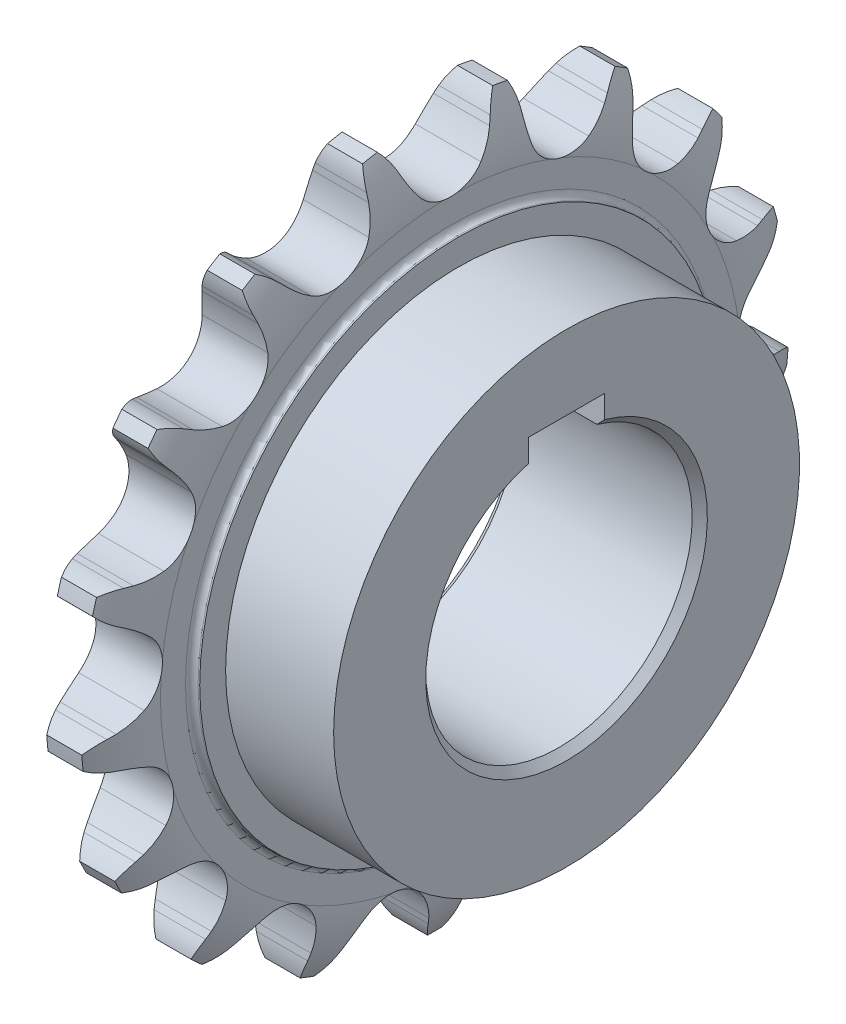
SolidWorks part; units mm, degrees
ref_plane "前视基准面" through (0, 0, 0) normal (0, 0, 1) x (1, 0, 0)
ref_plane "上视基准面" through (0, 0, 0) normal (0, 1, 0) x (1, 0, 0)
ref_plane "右视基准面" through (0, 0, 0) normal (1, 0, 0) x (0, 0, -1)
sketch "草图1" plane through (0, 0, 0) normal (0, 0, 1) x (1, 0, 0)
  line L0 (-7.9375, 0) -> (7.9375, 0) construction
  line L1 (-5.4059, 17.5) -> (-5.4059, 34)
  line L2 (-5.4059, 34) -> (-5.1989, 34)
  line L3 (-4.371, 34.8279) -> (-4.371, 38.1174)
  line L4 (-2.3072, 46.5) -> (2.3072, 46.5)
  line L5 (4.371, 38.1174) -> (4.371, 34.8279)
  line L6 (5.1989, 34) -> (5.4059, 34)
  line L7 (5.4059, 34) -> (5.4059, 17.5)
  line L8 (5.4059, 17.5) -> (-5.4059, 17.5)
  line L9 (0, 0) -> (0, 46.5) construction
  line L10 (-3.7169, 43.1974) -> (3.7169, 43.1974) construction
  line L11 (-3.7169, -43.1974) -> (3.7169, -43.1974) construction
  line L12 (7.9375, 0) -> (24.9375, 0) construction
  line L13 (-4.371, 38.1174) -> (3.7984, 38.1174) construction
  line L14 (-4.371, -38.1174) -> (3.7984, -38.1174) construction
  line L15 (24.9375, 0) -> (35.0975, 0) construction
  line L16 (35.0975, 0) -> (50.1875, 0) construction
  line L17 (50.1875, 0) -> (59.5875, 0) construction
  line L18 (59.5875, 0) -> (77.6975, 0) construction
  arc A0 (-2.3072, 46.5) -> (-4.371, 38.1174) centre (11.4948, 38.6567) ccw
  arc A1 (2.3072, 46.5) -> (4.371, 38.1174) centre (-11.4948, 38.6567) cw
  arc A2 (4.371, 34.8279) -> (5.1989, 34) centre (5.1989, 34.8279) ccw
  arc A3 (-5.1989, 34) -> (-4.371, 34.8279) centre (-5.1989, 34.8279) ccw
  point P30 (4.371, 34)
  point P33 (-4.371, 34)
  dimension "D1" = 4.1174
  dimension "rx" = 15.875
  dimension "D3" = 0.8279
  dimension "d" = 86.3948
  dimension "p" = 15.875
  dimension "z" = 17
  dimension "da" = 93
  dimension "df" = 76.2348
  dimension "dr" = 10.16
  dimension "dk" = 35
  dimension "dg" = 68
  dimension "h" = 15.09
  dimension "bf1" = 8.742
  dimension "b1" = 9.4
  dimension "ba" = 2.0638
  dimension "D2" = 1.0349
  dimension "pt" = 18.11
revolve "旋转1" add sketch "草图1" angle 360 about L0
sketch "草图2" plane through (0, 0, 0) normal (1, 0, 0) x (0, 0, -1)
  line L0 (0, 0) -> (0, 46.5) construction
  line L1 (0, 0) -> (-8.5444, 45.7082) construction
  line L2 (0, 0) -> (-16.7977, 43.36) construction
  line L3 (4.033, 39.986) -> (5.4737, 38.8388) construction
  line L4 (5.7931, 42.895) -> (-6.3584, 48.2605) construction
  line L5 (0, 0) -> (8.5444, 45.7082) construction
  line L6 (5.7931, 42.895) -> (6.1811, 43.7738)
  line L7 (-5.7931, 42.895) -> (-6.1811, 43.7738)
  circle A0 centre (0, 0) radius 46.5 construction
  arc A1 (4.033, 39.986) -> (-4.033, 39.986) centre (0, 43.1974) cw
  arc A2 (4.033, 39.986) -> (5.7931, 42.895) centre (-6.3584, 48.2605) ccw
  arc A3 (7.5795, 45.8781) -> (6.1811, 43.7738) centre (12.9831, 40.7704) ccw
  arc A4 (-4.033, 39.986) -> (-5.7931, 42.895) centre (6.3584, 48.2605) cw
  arc A5 (-7.5795, 45.8781) -> (-6.1811, 43.7738) centre (-12.9831, 40.7704) cw
  arc A7 (7.5795, 45.8781) -> (-7.5795, 45.8781) centre (0, 0) ccw
  dimension "r1" = 5.1554
  dimension "r3" = 7.4355
  dimension "D1" = 21.176
  dimension "D2" = 10.588
  dimension "α/2" = 51.471
  dimension "M" = 6.3584
  dimension "T" = 5.0631
  dimension "β" = 14.706
  dimension "γ/2" = 13.235
  dimension "bc" = 0.9606
extrude "切除-拉伸1" cut sketch "草图2" against normal mid plane 10.8118
pattern_circular "阵列(圆周)1" count 17 over 360 about axis through (0, 0, 0) along (1, 0, 0) of "切除-拉伸1"
sketch "草图3" plane through (0, 0, 0) normal (0, 0, 1) x (1, 0, 0)
  line L0 (5.4059, 17.5) -> (19.5941, 17.5)
  line L3 (19.5941, 17.5) -> (19.5941, 30.5973)
  line L4 (19.5941, 30.5973) -> (5.4059, 30.5973)
  line L5 (5.4059, 30.5973) -> (5.4059, 17.5)
  line L6 (0, 0) -> (6.4, 0) construction
  line L8 (-5.4059, 34) -> (-5.4059, -34) construction
  dimension "h" = 13.0973
  dimension "K" = 6.4
  dimension "L" = 25
revolve "旋转2" add sketch "草图3" angle 360 about L6
sketch "草图4" plane through (-5.4059, 0, 0) normal (-1, 0, 0) x (0, 0, 1)
  line L1 (-5, 16.7705) -> (5, 16.7705)
  line L2 (-5, 16.7705) -> (-5, 20.8)
  line L3 (-5, 20.8) -> (5, 20.8)
  line L4 (5, 16.7705) -> (5, 20.8)
  circle A0 centre (0, 0) radius 17.5 construction
  point P6 (1.7, 20.8)
  dimension "D1" = 20.8
  dimension "键槽宽度" = 10
  dimension "t1" = 3.3
extrude "切除-拉伸2" cut sketch "草图4" against normal through all
chamfer "倒角1" distance 1 angle 45 1 edges at (-5.4059, -17.5, 0)
chamfer "倒角2" distance 1 angle 45 1 edges at (19.5941, -17.5, 0)
